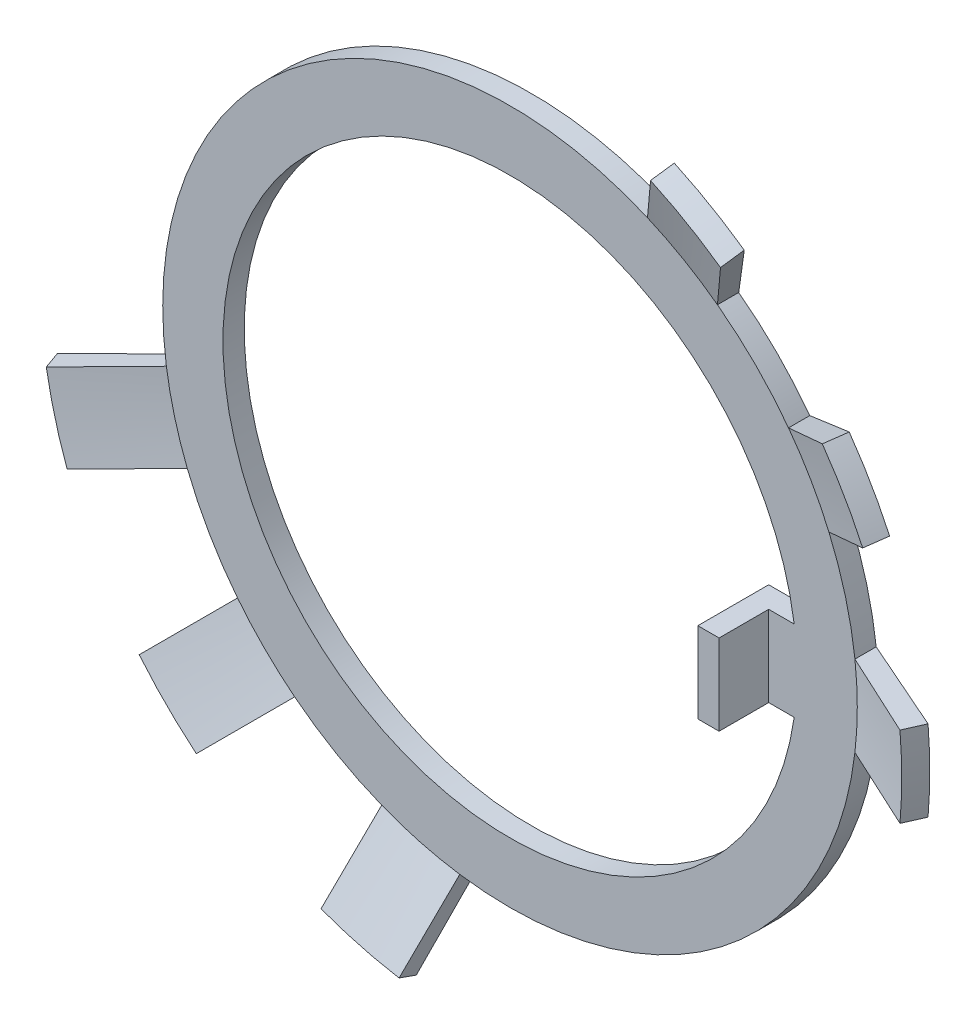
SolidWorks part; units mm, degrees
ref_plane "Front" through (0, 0, 0) normal (0, 0, 1) x (1, 0, 0)
ref_plane "Top" through (0, 0, 0) normal (0, 1, 0) x (1, 0, 0)
ref_plane "Right" through (0, 0, 0) normal (1, 0, 0) x (0, 0, -1)
other "Configuration Table"
sketch "Sketch1" plane through (0, 0, 0) normal (1, 0, 0) x (0, 1, 0)
  line L0 (0, -4.248) -> (-24.5, -4.248)
  line L1 (-24.5, -4.248) -> (-31, -1.3717)
  line L2 (0, 5.8236) -> (0, -8.1378) construction
  line L4 (-30.393, 0) -> (-24.5, -2.748)
  line L5 (-24.5, -2.748) -> (0, -2.748)
  line L6 (0, -2.748) -> (0, -4.248)
  line L7 (-31, -1.3717) -> (-30.393, 0)
revolve "Base-Extrude" add sketch "Sketch1" angle 360 about L2
sketch "Sketch2" plane through (-2.4044, 1.0036, -4.248) normal (0, 0, -1) x (-1, 0, 0)
  line L0 (-22.4528, 1.8464) -> (-19.1544, 1.8464)
  line L1 (-19.1544, 1.8464) -> (-19.1544, -3.8536)
  line L2 (-19.1544, -3.8536) -> (-22.4528, -3.8536)
  line L3 (-26.738, -3.8536) -> (-33.2731, -3.8536)
  line L4 (-26.738, 1.8464) -> (-33.2731, 1.8464)
  line L5 (-22.0529, 13.6314) -> (-27.7124, 16.899)
  line L6 (-24.9029, 8.6951) -> (-30.5624, 11.9626)
  line L7 (-12.103, 21.495) -> (-15.3705, 27.1545)
  line L8 (-17.0394, 18.645) -> (-20.3069, 24.3045)
  line L9 (-2.4044, 13.9688) -> (-2.4044, -17.023) construction
  line L10 (-2.4044, -1.0036) -> (1.5148, -15.6299) construction
  line L11 (1.1408, -25.2457) -> (2.8322, -31.5581)
  line L12 (6.6466, -23.7705) -> (8.3379, -30.0828)
  line L13 (16.8174, -16.1948) -> (21.4384, -20.8158)
  line L14 (12.7869, -20.2253) -> (17.4079, -24.8463)
  line L15 (21.8378, -4.5487) -> (28.1502, -6.2401)
  line L16 (20.3625, -10.0545) -> (26.6749, -11.7459)
  line L17 (-2.4044, -1.0036) -> (1.1408, -25.2457) construction
  arc A0 (-22.4528, -3.8536) -> (-22.4528, 1.8464) centre (-2.4044, -1.0036) ccw
  circle A1 centre (-2.4044, -1.0036) radius 24.5 construction
  arc A2 (-26.738, -3.8536) -> (1.1408, -25.2457) centre (-2.4044, -1.0036) ccw
  arc A4 (-27.7124, 16.899) -> (-30.5624, 11.9626) centre (-2.4044, -1.0036) ccw
  arc A5 (-17.0394, 18.645) -> (-22.0529, 13.6314) centre (-2.4044, -1.0036) ccw
  arc A6 (-24.9029, 8.6951) -> (-26.738, 1.8464) centre (-2.4044, -1.0036) ccw
  arc A7 (-33.2731, 1.8464) -> (-33.2731, -3.8536) centre (-2.4044, -1.0036) ccw
  arc A8 (-15.3705, 27.1545) -> (-20.3069, 24.3045) centre (-2.4044, -1.0036) ccw
  arc A9 (2.8322, -31.5581) -> (8.3379, -30.0828) centre (-2.4044, -1.0036) ccw
  arc A10 (17.4079, -24.8463) -> (21.4384, -20.8158) centre (-2.4044, -1.0036) ccw
  arc A11 (26.6749, -11.7459) -> (28.1502, -6.2401) centre (-2.4044, -1.0036) ccw
  arc A12 (21.8378, -4.5487) -> (-12.103, 21.495) centre (-2.4044, -1.0036) ccw
  arc A13 (16.8174, -16.1948) -> (20.3625, -10.0545) centre (-2.4044, -1.0036) ccw
  arc A14 (6.6466, -23.7705) -> (12.7869, -20.2253) centre (-2.4044, -1.0036) ccw
  circle A16 centre (-2.4044, -1.0036) radius 31 construction
extrude "Cut-Extrude" cut sketch "Sketch2" against normal through all flip side to cut
sketch "Sketch4" plane through (16.75, -0.6673, -0.255) normal (-1, 0, 0) x (0, 1, 0)
  line L1 (-2.1827, 2.4929) -> (3.5173, 2.4929)
  line L2 (-2.1827, 2.4929) -> (-2.1827, -1.0071)
  line L3 (-2.1827, -1.0071) -> (3.5173, -1.0071)
  line L4 (3.5173, 2.4929) -> (3.5173, -1.0071)
  line L8 (-2.1827, 2.4929) -> (3.5173, 2.4929) construction
  line L9 (3.5173, 2.4929) -> (3.5173, 3.9929) construction
  line L10 (-2.1827, 2.4929) -> (-2.1827, 3.9929) construction
  line L11 (3.5173, 3.9929) -> (-2.1827, 3.9929) construction
  dimension "h" = 5
extrude "Extrude1" add sketch "Sketch4" against normal blind 1.5
equation "\"D11@Sketch2\" = \"b@Sketch2\" / 2"
equation "\"D6@Sketch2\" = \"b@Sketch2\""
equation "\"D7@Sketch2\" = \"b@Sketch2\" / 2"
equation "\"S1@Sketch1\" = \"S@Sketch1\""
equation "\"b2@Sketch2\" = \"b@Sketch2\" / 2"
equation "\"b1@Sketch2\" = \"b@Sketch2\""
equation "\"D1@Extrude1\"=\"S@Sketch1\""
